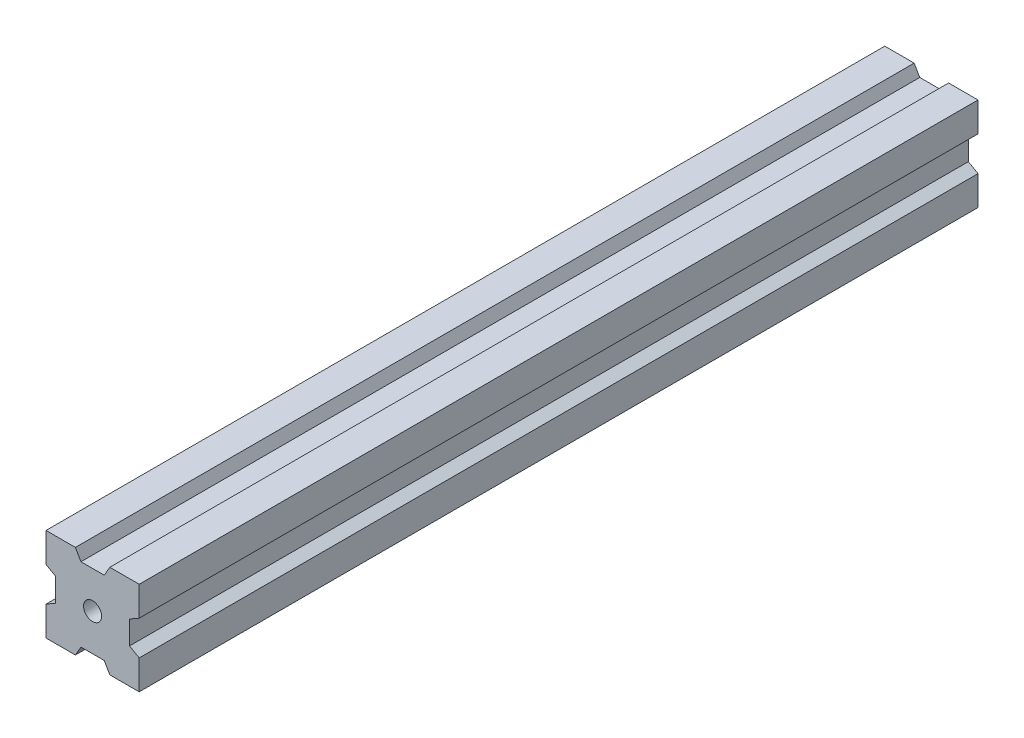
from build123d import *

# Parameters (mm, degrees)
SKETCH_1_W               = 20
SKETCH_1_H               = 20
SKETCH_1_R               = 1.94442565
EXTRUDE_1_DEPTH          = 90
CUT_EXTRUDE_1_DEPTH      = 181.554700853
PATTERN_CIRCULAR_1_COUNT = 4


with BuildPart() as part:
    # 草图1 → 凸台-拉伸1 (new, symmetric)
    with BuildSketch(Plane.XY):
        Rectangle(SKETCH_1_W, SKETCH_1_H)
        with Locations(Location((0, 0, 0), (0, 0, 180))):
            Circle(SKETCH_1_R, mode=Mode.SUBTRACT)
    extrude(amount=EXTRUDE_1_DEPTH, both=True)

    # 草图2 → 切除-拉伸1 (cut, symmetric)
    with BuildSketch(Plane.XY.offset(90)):
        Polygon((-32.933615203, 60.643738676), (-3.694439046, 10), (-2.5, 7.931170886), (2.5, 7.931170886), (3.694439046, 10), (32.933615203, 60.643738676), (32.933615203, 177.600443305), (-32.933615203, 177.600443305), align=None)
    cut_extrude_1 = extrude(amount=CUT_EXTRUDE_1_DEPTH, both=True, mode=Mode.SUBTRACT)

    # 阵列(圆周)1: 切除-拉伸1 ×4 about axis
    pattern_circular_1_axis = Axis((0, 0, 90), (0, 0, -1))
    for i in range(1, PATTERN_CIRCULAR_1_COUNT):
        add(cut_extrude_1.rotate(pattern_circular_1_axis, i * 360 / PATTERN_CIRCULAR_1_COUNT), mode=Mode.SUBTRACT)


solid = part.part
